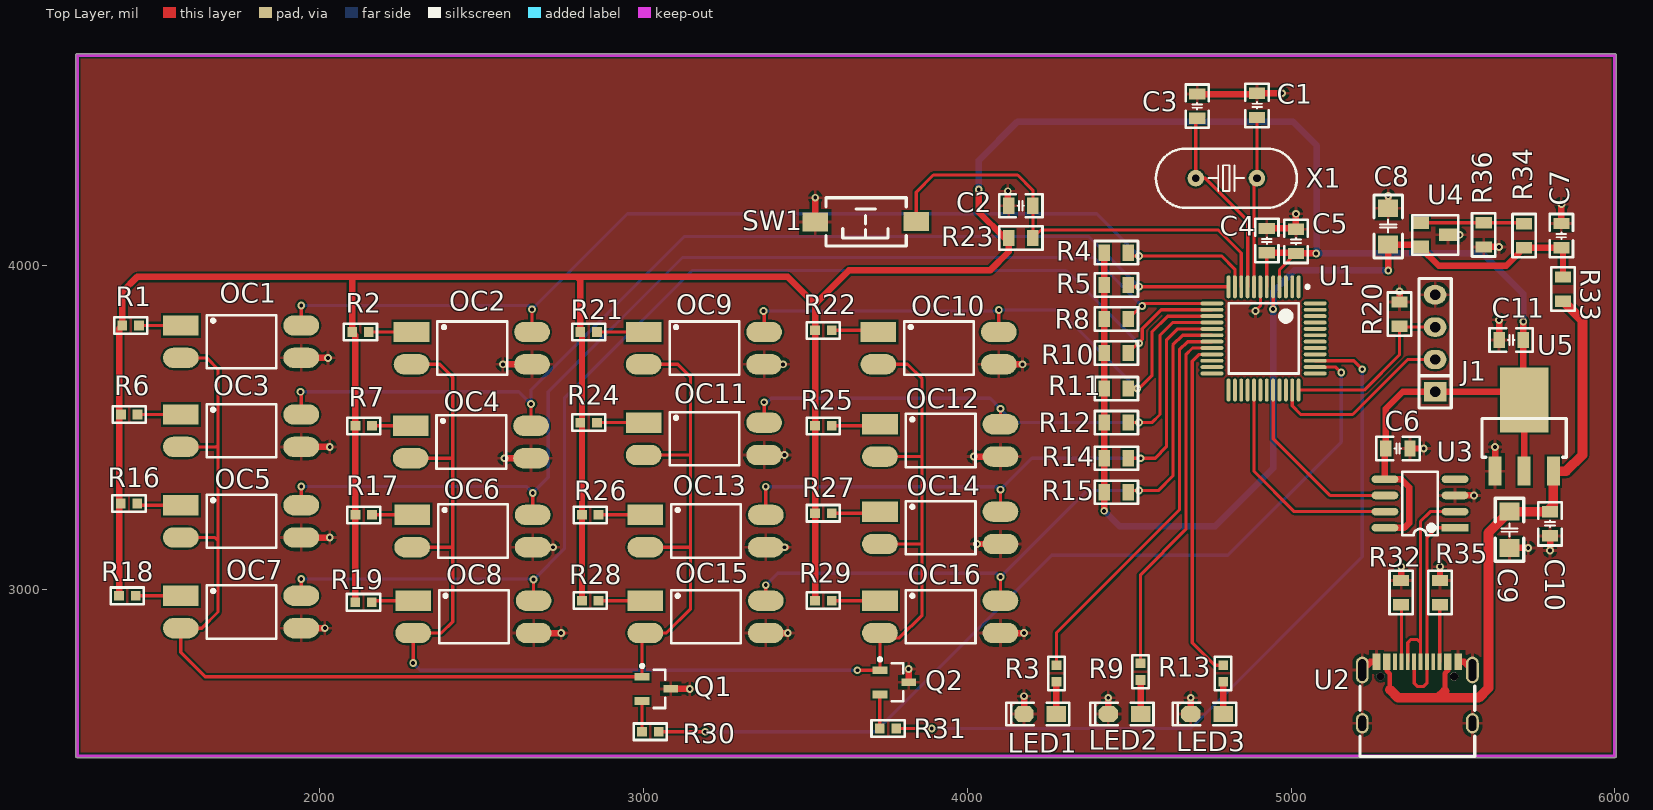
[diagram p0: Top Layer view]
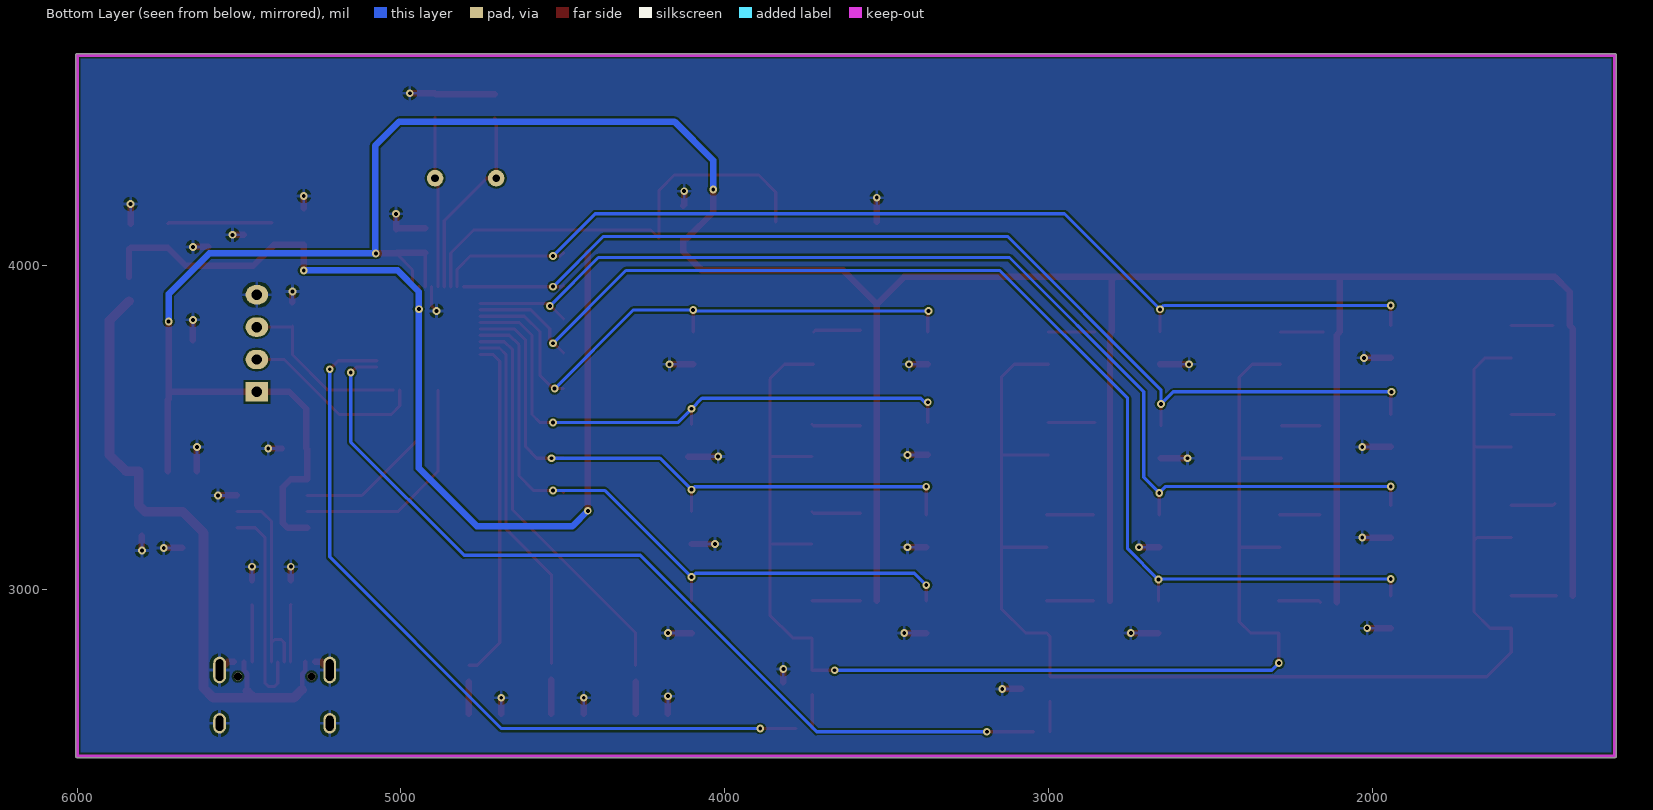
[diagram p1: Bottom Layer view, seen from below]
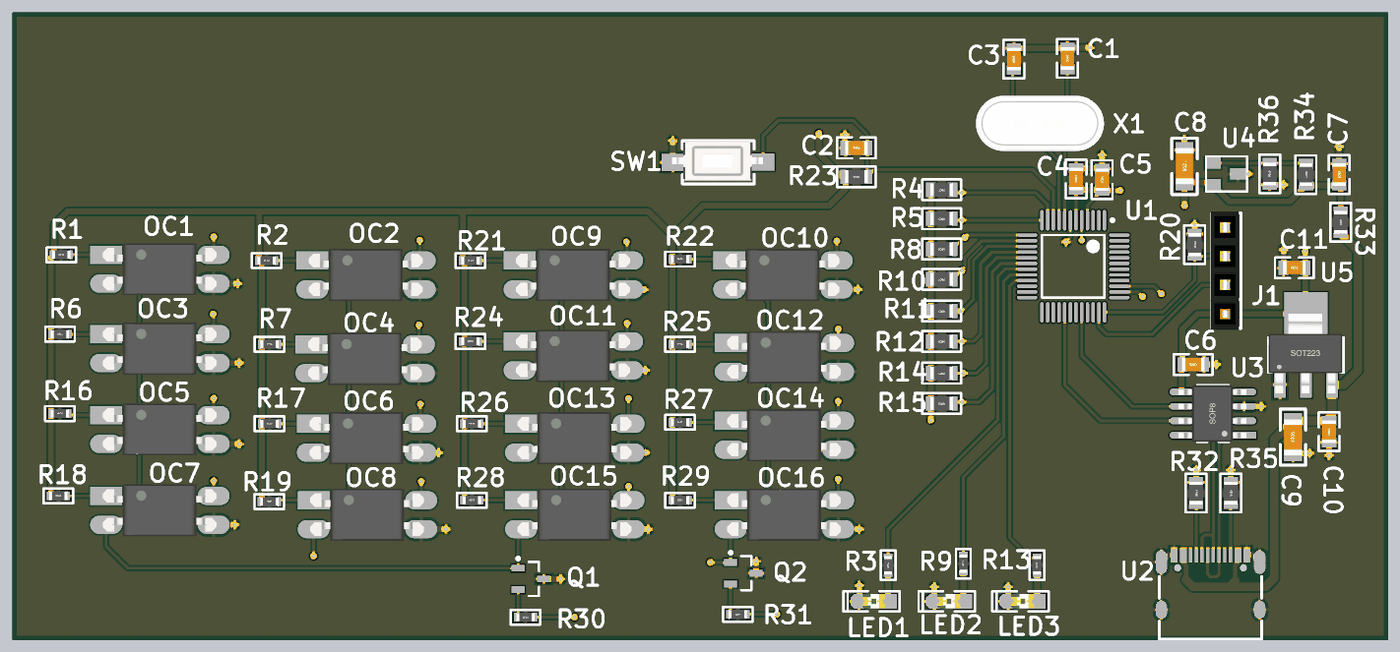
[diagram p2: 3D render of the assembled board from above, using the file's embedded part models]
# Altium PCB MISC82094.PcbDoc
Units mil, origin at the board's own origin, x right, y up, seen from the top; angles counter-clockwise.
Board outline 4760.03 x 2175.03 mil, 2 copper layers (Top Layer, Bottom Layer); 76 components, 52 nets, 259 pads, 75 vias.

## Layer stack, top to bottom (the 12.6 mil dielectric is the usual default, probably not edited)
Top Solder: solder mask 0.4, Solder Resist, Dk 3.5
Top Layer: signal copper 1.4
Dielectric 1: dielectric 12.6, FR-4, Dk 4.8
Bottom Layer: signal copper 1.4
Bottom Solder: solder mask 0.4, Solder Resist, Dk 3.5

## Board outline
1250,2479.99 cw(c1250,2485) 1244.98,2485 1244.98,4650 cw(c1250,4650) 1250,4655.02 6000,4655.02 cw(c6000,4650) 6005.02,4650 6005.02,2485 cw(c6000,2485) 6000,2479.99

## Design rules (kind name [scope] priority, off if disabled: settings)
Clearance [All] p1: gap=6
MinimumSolderMaskSliver [All] p1: minsoldermaskwidth=0
PolygonConnect [All] p1: connectstyle=Relief reliefconductorwidth=10 reliefentries=4 polygonreliefangle="90 Angle" airgapwidth=10
RoutingVias [All] p1: holewidth=28 width=50 viastyle="Through Hole" minholewidth=28 minwidth=50 maxholewidth=28 maxwidth=50
SilkToSilkClearance [All] p1: silktosilkclearance=0
SilkToSolderMaskClearance [IsPad] p1: minsilkscreentomaskgap=0 clearancetoexposedcopper=TRUE
SolderMaskExpansion [All] p1: expansion=4
Width [All] p1: maxlimit=50 minlimit=10 preferedwidth=10
27 further rules are at their usual default settings.

## Components (designator, comment, footprint, x,y, rotation, side; value= is the part's Value field where it differs from the comment)
C1 "22PF" "C 0805_L" 4895,4495 r270 top
C2 "0.1UF" "C 0805_L" 4165,4185 r0 top
C3 "22PF" "C 0805_L" 4710,4492.6 r90 top
C4 "0.1UF" "C 0805_L" 4925,4077.4 r270 top
C5 "0.1UF" "C 0805_L" 5015,4075 r270 top
C6 "0.1UF" "C 0805_L" 5330,3435 r180 top
C7 "0.1UF" "C 0805_L" 5835,4092.6 r270 top
C8 "10UF" "C 1206_L" 5300,4122.09 r270 top
C9 "30UF" "C 1206_L" 5675,3182.91 r90 top
C10 "0.1UF" "C 0805_L" 5800,3202.4 r90 top
C11 "0.1UF" "C 0805_L" 5680,3770 r0 top
J1 "Female HDR1X4" Fe-HDR1X4/2.54-S 5445,3610 r180 top
LED1 "Red" "LED 0805G" 4225,2615 r180 top
LED2 "Red" "LED 0805G" 4485,2615 r180 top
LED3 "Red" "LED 0805G" 4740,2615 r180 top
OC1 "ITR20001" SMD_PC817 1570,3815 r0 top
OC2 "ITR20001" SMD_PC817 2282.88,3795 r0 top
OC3 "ITR20001" SMD_PC817 1570,3540 r0 top
OC4 "ITR20001" SMD_PC817 2280,3505 r0 top
OC5 "ITR20001" SMD_PC817 1570,3260 r0 top
OC6 "ITR20001" SMD_PC817 2285,3230 r0 top
OC7 "ITR20001" SMD_PC817 1570,2980 r0 top
OC8 "ITR20001" SMD_PC817 2287.88,2965 r0 top
OC9 "ITR20001" SMD_PC817 3000,3795 r0 top
OC10 "ITR20001" SMD_PC817 3725,3795 r0 top
OC11 "ITR20001" SMD_PC817 3000,3515 r0 top
OC12 "ITR20001" SMD_PC817 3730,3510 r0 top
OC13 "ITR20001" SMD_PC817 3005,3230 r0 top
OC14 "ITR20001" SMD_PC817 3730,3240 r0 top
OC15 "ITR20001" SMD_PC817 3005,2965 r0 top
OC16 "ITR20001" SMD_PC817 3730,2965 r0 top
Q1 "QNPN" SOT-23B_N 3039.29,2692.4 r0 top
Q2 "QNPN" SOT-23B_N 3774.29,2712.6 r0 top
R1 "330" "R 0603_L" 1415,3815 r0 top
R2 "330" "R 0603_L" 2125,3795 r0 top
R3 "330" "R 0603_L" 4275,2740 r90 top
R4 "10K" "R 0805_L" 4460,4040 r180 top
R5 "10K" "R 0805_L" 4460,3940 r180 top
R6 "330" "R 0603_L" 1410.59,3540 r0 top
R7 "330" "R 0603_L" 2135,3505 r0 top
R8 "10K" "R 0805_L" 4460,3835 r180 top
R9 "330" "R 0603_L" 4535,2745.59 r90 top
R10 "10K" "R 0805_L" 4460,3730 r180 top
R11 "10K" "R 0805_L" 4460,3620 r180 top
R12 "10K" "R 0805_L" 4460,3515 r180 top
R13 "330" "R 0603_L" 4790,2740 r90 top
R14 "10K" "R 0805_L" 4460,3405 r180 top
R15 "10K" "R 0805_L" 4460,3300 r180 top
R16 "330" "R 0603_L" 1410,3265 r0 top
R17 "330" "R 0603_L" 2135,3230 r0 top
R18 "330" "R 0603_L" 1405,2980 r0 top
R19 "330" "R 0603_L" 2134.41,2960 r0 top
R20 "10K" "R 0805_L" 5335,3850 r270 top
R21 "330" "R 0603_L" 2830,3795 r0 top
R22 "330" "R 0603_L" 3555,3800 r0 top
R23 "10K" "R 0805_L" 4165,4085 r180 top
R24 "330" "R 0603_L" 2830,3515 r0 top
R25 "330" "R 0603_L" 3555,3505 r0 top
R26 "330" "R 0603_L" 2835,3230 r0 top
R27 "330" "R 0603_L" 3555,3235 r0 top
R28 "330" "R 0603_L" 2835,2965 r0 top
R29 "330" "R 0603_L" 3555,2965 r0 top
R30 "330" "R 0603_L" 3020.59,2560 r180 top
R31 "330" "R 0603_L" 3755,2570 r180 top
R32 "5.1K" "R 0805_L" 5340,2990 r270 top
R33 "330" "R 0805_L" 5840,3927.6 r270 top
R34 "3.3K" "R 0805_L" 5720,4092.4 r270 top
R35 "5.1K" "R 0805_L" 5460,2990 r270 top
R36 "10K" "R 0805_L" 5595,4095 r90 top
SW1 "3x6x5" "TSW SMD-3*6*2.5" 3685,4135 r180 top
U1 "STM32G030C8T6" LQFP48_N 4915,3775 r270 top
U2 "HC-TYPE-C-16P-01A COPY" USB-C-SMD_HC-TYPE-C-16P-01A 5390,2640 r0 top
U3 "CH340N" SOP8 5506.54,3190 r180 top
U4 "TL431DBZ" SOT-23 5445.63,4095 r270 top
U5 "AMS1117" SOT223 5720,3365 r0 top
X1 "12MHz" "OSC HC-49S" 4800,4270 r0 top

## Footprints (in the part's own frame and the unit in brackets; to place one, negate y for a bottom-side part, rotate by r counter-clockwise, add the part's x,y. Pads: shape width x height; smd on the part's side, far side on the other; paste and mask are expansions set on the pad)
"C 0805_L" [mil] "无极性贴片电容"
  rect 35x50 smd: 1(-37.4,0) 2(37.4,0)
  silkscreen extent -67,-36 67,36, body extent -39,-24 39,24, height 20
"C 1206_L" [mil] "无极性贴片电容"
  rect 55x62 smd: 1(-55.12,0) 2(57.09,0)
  silkscreen extent -96,-44 98,44, body extent -63,-32 63,32, height 48
Fe-HDR1X4/2.54-S [mil]
  rect 70x60 hole 32: 1(0,0)
  oval 70x60 hole 32: 2(0,-100) 3(0,-200) 4(0,-300)
  silkscreen extent -50,-350 50,50, body extent -44,-355 54,55, height 335
"LED 0805G" [mil] "绿色0805LED"
  rect 60x50 smd: 1(-50,0)
  oct 60x50 smd: 2(50,0)
  silkscreen extent -90,-35 105,35, body extent -39,-25 39,25, height 32
LQFP48_N [mm] "Thin QFP, 48-Leads, Body 7x7mm, Pitch 0.5mm, IPC Medium Density"
  oval 1.8x0.3 smd: 1(-4.05,2.75) 2(-4.05,2.25) 3(-4.05,1.75) 4(-4.05,1.25) 5(-4.05,0.75) 6(-4.05,0.25) 7(-4.05,-0.25) 8(-4.05,-0.75) 9(-4.05,-1.25) 10(-4.05,-1.75) 11(-4.05,-2.25) 12(-4.05,-2.75) 25(4.05,-2.75) 26(4.05,-2.25) 27(4.05,-1.75) 28(4.05,-1.25) 29(4.05,-0.75) 30(4.05,-0.25) 31(4.05,0.25) 32(4.05,0.75) 33(4.05,1.25) 34(4.05,1.75) 35(4.05,2.25) 36(4.05,2.75)
  oval 0.3x1.8 smd: 13(-2.75,-4.05) 14(-2.25,-4.05) 15(-1.75,-4.05) 16(-1.25,-4.05) 17(-0.75,-4.05) 18(-0.25,-4.05) 19(0.25,-4.05) 20(0.75,-4.05) 21(1.25,-4.05) 22(1.75,-4.05) 23(2.25,-4.05) 24(2.75,-4.05) 37(2.75,4.05) 38(2.25,4.05) 39(1.75,4.05) 40(1.25,4.05) 41(0.75,4.05) 42(0.25,4.05) 43(-0.25,4.05) 44(-0.75,4.05) 45(-1.25,4.05) 46(-1.75,4.05) 47(-2.25,4.05) 48(-2.75,4.05)
  silkscreen extent -4.17,-2.75 2.75,3.58, body extent -3.5,-3.5 3.5,3.5, height 1.6
"OSC HC-49S" [mm]
  round 1.3 hole 0.6: 1(-2.4,0) 2(2.4,0)
  silkscreen extent -5.52,-2.32 5.52,2.33, body extent -5.52,-2.32 5.53,2.33, height 4.13
"R 0603_L" [mil] "1/10W贴片电阻"
  rect 30x30 smd: 1(-25.59,0) 2(25.59,0)
  silkscreen extent -51,-26 51,26, body extent -31,-16 32,16, height 16
"R 0805_L" [mil] "1/8W贴片电阻"
  rect 35x50 smd: 1(-37.4,0) 2(37.4,0)
  silkscreen extent -67,-36 67,36, body extent -39,-25 39,25, height 20
SMD_PC817 [mm]
  rect 2.8x1.6 smd mask+0: 1(0,0)
  oval 2.8x1.6 smd mask+0: 2(0,-2.54) 3(9.452,-2.54) 4(9.452,0)
  silkscreen extent 2.03,-3.36 7.49,0.82, body extent -0.3,-3.56 9.7,1.02, height 3.85
SOP8 [mm]
  rect 2.1x0.6 smd: 1(0,0)
  oval 2.1x0.6 smd: 2(0,-1.27) 3(0,-2.54) 4(0,-3.81) 5(5.5,-3.81) 6(5.5,-2.54) 7(5.5,-1.27) 8(5.5,0)
  silkscreen extent 1.35,-4.41 4.15,0.6, body extent -0.21,-4.4 5.8,0.6, height 1.9
SOT223 [mil]
  rect 40x90 smd: 1(-90,0) 2(0,0) 3(90,0)
  rect 150x200 smd: 2(0,220)
  silkscreen extent -130,43 130,163, body extent -130,-30 126,246, height 65
SOT-23 [mm]
  rect 1x1.4 smd paste+0 mask+0.051: 1(-0.95,-1.2) 2(0.95,-1.2) 3(0,1)
  silkscreen extent -1.55,-1.8 1.55,1.8
SOT-23B_N [mm] "SOT23, 3-Leads, Body 2.9x1.3mm, Pitch 0.95mm, Lead Span 2.4mm, IPC Medium Density"
  rect 1.15x0.6 smd: 1(-1.125,0.95) 2(-1.125,-0.95) 3(1.125,0)
  silkscreen extent -1.25,-1.5 0.7,1.92, body extent -0.7,-1.5 0.7,1.5, height 1.14
"TSW SMD-3*6*2.5" [mm] "3*6*2.5mm"
  rect 2x1.5 smd: 1(-3.996,-0.02) 2(3.937,0)
  silkscreen extent -3.21,-1.9 3.09,1.9, body extent -4,-1.88 4,1.62, height 2.59
USB-C-SMD_HC-TYPE-C-16P-01A [mm]
  oval 1x2.1 hole 0.6 slot 1.7 at 90 deg paste+0 mask+0.05: 1(-4.32,2.809) 2(4.32,2.809)
  oval 1x1.6 hole 0.6 slot 1.2 at 90 deg paste+0 mask+0.05: 3(4.32,-1.372) 4(-4.32,-1.372)
  rect 0.6x1.3 smd paste-100 mask+0.05: A1B12(-3.2,3.448) A4B9(-2.4,3.448) B1A12(3.2,3.448) B4A9(2.4,3.448)
  rect 0.3x1.3 smd paste-100 mask+0.05: A5(-1.25,3.448) A6(-0.25,3.448) A7(0.25,3.448) A8(1.25,3.448) B5(1.75,3.448) B6(0.75,3.448) B7(-0.75,3.448) B8(-1.75,3.448)
  round 0.65 hole 0.65 unplated paste+0: ""(-2.89,2.308) ""(2.89,2.308)
  silkscreen extent -4.5,-3.97 4.5,1.55

## Part data
C1 C2 C3 C4 C5 C6 C7 C8 C9 C10 C11: library part C, "SMD capacitor"
LED1 LED2 LED3: library part LED-SMD, "SMD LED"
OC1 OC2 OC3 OC4 OC5 OC6 OC7 OC8 OC9 OC10 OC11 OC12 OC13 OC14 OC15 OC16: library part PC817, "Linear optocoupler"
Q1 Q2: "NPN Bipolar Transistor"
R1 R2 R3 R4 R5 R6 R7 R8 R9 R10 R11 R12 R13 R14 R15 R16 R17 R18 R19 R20 R21 R22 R23 R24 R25 R26 R27 R28 R29 R30 R31 R32 R33 R34 R35 R36: library part R, "SMD resistor"
SW1: library part "TSW 3x6", "3x6 tact switch"
U5: "Three-terminal voltage regulator"
X1: library part XTAL-2P, "2-pin passive crystal oscillator"

## Via types
v1: diameter 24, hole 12, Top Layer to Bottom Layer, 75 vias

## Nets (pads, with @x,y where several pads share a name; then routed paths per layer and width w, separated by ;. In a path a pad name is that pad's centre, name@x,y a point inside that pad or via, vN(x,y) a via of type N, cw(c..) or ccw(c..) an arc to the next point about the centre after c; other vN are vias at no path point)
ADC_IN0: OC1.4 OC2.4 R4.1 U1.11 | length 3305.5
  Top Layer w10: OC1.4 v1(1942.12,3877.12) ; OC2.4 v1(2655,3865) ; R4.1 4507.41,4030 v1(4530,4030) 4785,4030 4826.42,3988.58 U1.11
  Bottom Layer w10: v1(1942.12,3877.12) 2642.88,3877.12 v1(2655,3865) 2950,4160 4400,4160 v1(4530,4030)
ADC_IN1: OC3.4 OC4.4 R5.1 U1.12 | length 3357.4
  Top Layer w10: OC3.4 v1@1942.12,3607.88 ; OC4.4 v1(2652.12,3572.12) ; R5.1 4502.96,3934.45 U1.12
  Bottom Layer w10: v1(1940,3610) 2614.24,3610 v1(2652.12,3572.12) 2652.12,3617.12 3125,4090 4375,4090 v1(4530,3935)
ADC_IN2: OC5.4 OC6.4 R8.1 U1.13 | length 3528.2
  Top Layer w10: OC5.4 v1(1942.12,3317.88) ; OC6.4 v1(2657.12,3297.88) ; R8.1 4545.67,3883.27 U1.13
  Bottom Layer w10: v1(1942.12,3317.88) 2637.12,3317.88 v1(2657.12,3297.88) 2705,3345.76 2705,3610 3120,4025 4390,4025 v1(4540,3875)
ADC_IN3: OC7.4 OC8.4 R10.1 U1.14 | length 3799.5
  Top Layer w10: OC7.4 v1(1942.12,3032.12) ; OC8.4 v1(2660,3030) ; R10.1 4540,3772.6 4540,3805 4598.58,3863.58 U1.14
  Bottom Layer w10: v1(1942.12,3032.12) 2657.88,3032.12 v1(2660,3030) 2755,3125 2755,3590 3150,3985 4305,3985 v1(4530,3760)
ADC_IN4: OC9.4 OC10.4 R11.1 U1.15 | length 1817.5
  Top Layer w10: OC9.4 v1@3372.12,3857.88 ; OC10.4 v1(4097.12,3862.88) ; R11.1 4530,3620 4570,3660 4570,3795 4618.9,3843.9 U1.15
  Bottom Layer w10: v1(3370,3860) 4094.24,3860 v1(4097.12,3862.88) 4282.12,3862.88 v1(4525,3620)
ADC_IN5: OC11.4 OC12.4 R12.1 U1.16 | length 1834.5
  Top Layer w10: OC11.4 v1(3372.12,3577.88) ; OC12.4 v1(4102.12,3557.88) ; R12.1 4570,3515 4595,3540.01 4595,3785 4634.21,3824.21 U1.16
  Bottom Layer w10: v1(3372.12,3577.88) 3382.12,3577.88 3394.24,3590 4070,3590 v1(4102.12,3557.88) 4145,3515 v1(4530,3515)
ADC_IN6: OC13.4 OC14.4 R14.1 U1.17 | length 1973.9
  Top Layer w10: OC13.4 v1(3377.12,3317.12) ; OC14.4 v1(4102.12,3307.88) ; R14.1 4580,3405 4615,3440 4615,3770 4649.53,3804.53 U1.17
  Bottom Layer w10: v1(3377.12,3317.12) 4092.88,3317.12 v1(4102.12,3307.88) 4199.24,3405 v1(4535,3405)
ADC_IN7: OC15.4 OC16.4 R15.1 U1.18 | length 2100.9
  Top Layer w10: OC15.4 v1(3377.12,3012.88) ; OC16.4 v1(4102.12,3037.88) ; R15.1 4502.4,3305 v1(4530,3305) 4590,3305 4635,3350 4635,3755 4664.84,3784.84 U1.18
  Bottom Layer w10: v1(3377.12,3012.88) 3414.24,3050 4090,3050 v1(4102.12,3037.88) 4369.24,3305 v1(4530,3305)
BANK0: R30.1 U1.38 | length 2781.9
  Top Layer w10: R30.1 v1(3190,2560) ; U1.38 5138.58,3686.42 v1(5155,3670)
  Bottom Layer w10: v1(3190,2560) 3715,2560 4260,3105 4805,3105 5155,3455 v1(5155,3670)
BANK1: R31.1 U1.39 | length 2395.3
  Top Layer w10: R31.1 v1(3890,2570) ; U1.39 5193.9,3706.1 v1(5220,3680)
  Bottom Layer w10: v1(3890,2570) 4690,2570 5220,3100 v1(5220,3680)
GND: C1.1 C2.1 C3.2 C4.1 C5.1 C6.1 C7.1 C8.1 C9.1 C10.1 C11.1 J1.4 LED1.2 LED2.2 LED3.2 OC1.3 OC2.3 OC3.3 OC4.3 OC5.3 OC6.3 OC7.3 OC8.3 OC9.3 OC10.3 OC11.3 OC12.3 OC13.3 OC14.3 OC15.3 OC16.3 Q1.3 Q2.3 R20.1 R32.1 R35.1 R36.1 SW1.2 U1.7 U2.1 U2.2 U2.3 U2.4 U2.A1B12 U2.B1A12 U3.3 U4.3 U5.1 | length 2825.1
  Top Layer w10: v1(4890,3860) 4905.16,3875.16 U1.7
  Top Layer w20: OC7.3 v1(2015,2880) ; OC5.3 v1(2030,3160) ; OC3.3 v1(2030,3440) ; OC1.3 v1(2025,3715) ; v1(2565,3695) OC2.3 ; v1(2570,3405) OC4.3 ; OC6.3 v1(2720,3130) ; OC8.3 v1@2750,2865 ; Q1.3 v1(3142.4,2692.4) ; OC11.3 v1(3435,3415) ; OC9.3 v1(3430,3695) ; OC15.3 v1(3445,2865) ; OC13.3 v1@3440,3130 ; SW1.2 v1(3530,4210) ; Q2.3 v1(3818.58,2753.58) ; v1(4020,3410) OC12.3@4112.12,3410 ; v1(4030,3140) OC14.3 ; OC10.3 v1(4170,3695) ; OC16.3 v1(4175,2865) ; v1(4125,4230) 4125,4187.59 C2.1 ; LED1.2 v1(4175,2670) ; LED2.2 v1(4435,2665) ; LED3.2 v1(4690,2665) ; C3.2 4892.59,4530 C1.1 v1(4972.4,4532.4) ; C4.1 5012.6,4114.8 C5.1 v1(5015,4160) ; U2.1 5245.1,2775.76 U2.A1B12 ; C8.1 v1(5300,4215) ; R20.1 v1(5335,3920) ; R32.1 v1(5340,3070) ; C6.1 v1(5410,3435) ; R35.1 v1(5460,3070) ; U4.3 v1(5520,4095) ; U3.3 v1(5565,3290) ; U2.B1A12 5534.89,2775.76 U2.2 ; R36.1 v1(5642.6,4057.6) ; U5.1 v1(5630,3440) ; C11.1 v1(5642.6,3832.4) ; C9.1 v1(5732.8,3127.8) ; v1(5800,3120) C10.1 ; C7.1 v1(5835,4190)
  other v1: 2745,2865 3435,3130
NetC1_2: C1.2 U1.8 X1.2 | length 527.1
  Top Layer w10: U1.8 4885.47,4260.98 X1.2 4894.49,4457.09 C1.2
NetC2_2: C2.2 R23.1 SW1.1 U1.10 | length 1428.6
  Top Layer w10: SW1.1 3842.31,4227.31 3895,4280 4155,4280 4202.4,4232.6 R23.1 4227.4,4110 4775,4110 4846.1,4038.9 U1.10
NetC3_1: C3.1 U1.9 X1.1 | length 606.3
  Top Layer w10: C3.1 4705.51,4450.71 X1.1 4735,4270 4865.79,4139.21 U1.9
NetLED1_1: LED1.1 R3.1 | length 99.4
  Top Layer w20: LED1.1 R3.1
NetLED2_1: LED2.1 R9.1 | length 105
  Top Layer w20: LED2.1 R9.1
NetLED3_1: LED3.1 R13.1 | length 99.4
  Top Layer w20: LED3.1 R13.1
NetOC1_1: OC1.1 R1.2 | length 129.4
  Top Layer w10: R1.2 OC1.1
NetOC1_2: OC1.2 OC3.2 OC5.2 OC7.2 OC9.2 OC11.2 OC13.2 OC15.2 Q1.1 | length 4256.6
  Top Layer w10: OC5.2 1675,3160 1685,3150 ; OC3.2 1680,3440 1685,3445 ; OC1.2 1650,3715 1685,3680 1685,3445 ; OC11.2 3145,3415 ; OC9.2 3105,3695 3145,3655 3145,3415 ; OC13.2 3140,3130 3145,3135 ; 1685,3150 1685,3445 ; 1685,3150 1685,2930 1635,2880 OC7.2 1570,2805 1645.2,2729.8 Q1.1 2995,2855 OC15.2 3070,2865 3145,2940 3145,3135 ; 3145,3135 3145,3415
NetOC2_1: OC2.1 R2.2 | length 132.3
  Top Layer w10: R2.2 OC2.1
NetOC2_2: OC2.2 OC4.2 OC6.2 OC8.2 OC10.2 OC12.2 OC14.2 OC16.2 Q2.1 | length 4241.2
  Top Layer w10: OC4.2 2405,3405 2410,3410 ; OC2.2 2370,3695 2410,3655 2410,3410 ; OC6.2 2410,3130 ; v1(2287.88,2772.12) OC8.2 2375,2865 2410,2900 2410,3130 ; v1(3660,2750) Q2.1 3730,2850 3790,2850 3860,2920 3860,3140 ; OC10.2 3815,3695 3860,3650 3860,3415 ; OC14.2 3860,3140 ; OC12.2 3855,3410 3860,3415 ; 2410,3130 2410,3410 ; 3860,3140 3860,3415
  Bottom Layer w10: v1(2287.88,2772.12) 2310,2750 v1(3660,2750)
NetOC3_1: OC3.1 R6.2 | length 133.8
  Top Layer w10: R6.2 OC3.1
NetOC4_1: OC4.1 R7.2 | length 119.4
  Top Layer w10: R7.2 OC4.1
NetOC5_1: OC5.1 R16.2 | length 136.5
  Top Layer w10: R16.2 1440.58,3260 OC5.1
NetOC6_1: OC6.1 R17.2 | length 124.4
  Top Layer w10: R17.2 OC6.1
NetOC7_1: OC7.1 R18.2 | length 139.4
  Top Layer w10: R18.2 OC7.1
NetOC8_1: OC8.1 R19.2 | length 130
  Top Layer w10: R19.2 2165,2965 OC8.1
NetOC9_1: OC9.1 R21.2 | length 144.4
  Top Layer w10: R21.2 OC9.1
NetOC10_1: OC10.1 R22.2 | length 146.5
  Top Layer w10: R22.2 3720,3800 OC10.1
NetOC11_1: OC11.1 R24.2 | length 144.4
  Top Layer w10: R24.2 OC11.1
NetOC12_1: OC12.1 R25.2 | length 151.5
  Top Layer w10: R25.2 3725,3505 OC12.1
NetOC13_1: OC13.1 R26.2 | length 144.4
  Top Layer w10: R26.2 OC13.1
NetOC14_1: OC14.1 R27.2 | length 151.5
  Top Layer w10: R27.2 3725,3235 OC14.1
NetOC15_1: OC15.1 R28.2 | length 144.4
  Top Layer w10: R28.2 OC15.1
NetOC16_1: OC16.1 R29.2 | length 149.4
  Top Layer w10: R29.2 OC16.1
NetQ1_2: Q1.2 R30.2 | length 95
  Top Layer w10: R30.2 Q1.2
NetQ2_2: Q2.2 R31.2 | length 105.4
  Top Layer w10: R31.2 3729.41,2674.61 Q2.2
NetR3_2: R3.2 U1.19 | length 1242.8
  Top Layer w10: R3.2 4275,2865 4655,3245 4655,3740 4680.16,3765.16 U1.19
NetR9_2: R9.2 U1.20 | length 1100.8
  Top Layer w10: R9.2 4535,3045 4675,3185 4675,3725 4695.47,3745.47 U1.20
NetR13_2: R13.2 U1.21 | length 1062.9
  Top Layer w10: U1.21 4715.79,3725.79 4695,3705 4695,2835 4764.41,2765.59 R13.2
NetR32_2: R32.2 U2.A5 | length 177.2
  Top Layer w10: R32.2 5340.79,2951.81 U2.A5
NetR34_1: R34.1 R36.2 U4.1 | length 322.7
  Top Layer w10: U4.1 R36.2 5717.4,4132.4 R34.1
NetR35_2: R35.2 U2.B5 | length 177.3
  Top Layer w10: U2.B5 5458.9,2951.5 R35.2
NetU2_A6: U2.A6 U2.B6 U3.1 | length 662.9
  Top Layer w10: U2.A6 5380.16,2709.84 5390,2700 5410,2700 5419.53,2709.53 U2.B6 5419.53,3159.53 5450,3190 U3.1
NetU2_A7: U2.A7 U2.B7 U3.2 | length 660.4
  Top Layer w10: U2.B7 5360.47,2835.47 5370,2845 5390,2845 5399.84,2835.16 ; U2.A7 5399.84,2835.16 ; U3.2 5430,3240 5399.84,3209.84 5399.84,2835.16
SWCLK: J1.3 R20.2 U1.36 | length 555.7
  Top Layer w10: U1.36 5225.55,3615.55 5335,3725 R20.2 5337.6,3810 J1.3
SWDIO: J1.2 U1.35 | length 571.9
  Top Layer w10: U1.35 5003.58,3566.42 5030,3540 5190,3540 5360,3710 J1.2
UART_RX: U1.32 U3.6 | length 568.2
  Top Layer w10: U1.32 4944.53,3465.47 5120,3290 U3.6
UART_TX: U1.29 U3.7 | length 707.1
  Top Layer w10: U1.29 4885.47,3364.53 5010,3240 U3.7
VBUS: C9.2 C10.2 R33.2 U2.A4B9 U2.B4A9 U5.3 | length 1971.4
  Top Layer w15: U2.A4B9 5295.51,2748.78 5305,2739.29 5305,2690 ; 5475,2685 5475,2740 5484.49,2749.49 U2.B4A9
  Top Layer w30: 5305,2690 5330,2665 5455,2665 ; 5475,2685 5455,2665 ; R33.2 5900,3830.2 5900,3415 5850,3365 U5.3 5810,3260 5790,3240 C9.2 5610,3175 5610,2695 5580,2665 5455,2665
VCC: C4.2 C5.2 C6.2 C11.2 J1.1 R1.1 R2.1 R6.1 R7.1 R16.1 R17.1 R18.1 R19.1 R21.1 R22.1 R23.2 R24.1 R25.1 R26.1 R27.1 R28.1 R29.1 U1.4 U1.6 U3.5 U3.8 U5.2 | length 11088
  Top Layer w10: U1.6 4924.84,4039.84 C4.2 ; U1.4 4964.21,3986.82 C5.2
  Top Layer w20: R18.1 1379.41,3805 R1.1 1389.41,3919.41 1435,3965 2095,3965 ; R19.1 2108.82,3785.58 R2.1 2099.41,3960.59 2095,3965 ; R28.1 R26.1 2809.41,3790 R21.1 2804.41,3955.59 2795,3965 ; R29.1 R27.1 R25.1 R22.1 3529.41,3880.59 ; v1(4035,4235) 4035,4165 4115,4085 R23.2 4127.6,4042.6 4070,3985 3633.81,3985 3529.41,3880.59 ; C4.2 5012.6,4040 C5.2 v1(5077.4,4037.6) ; U3.8 5350.3,3190 5365,3204.7 5365,3315 5340,3340 U3.5 5290,3432.4 C6.2 5292.6,3557.6 5345,3610 J1.1 U5.2@5717.4,3610 ; v1(5717.4,3827.4) C11.2 U5.2@5717.4,3610 ; U5.2@5720,3365 5720,3585 5717.4,3587.6 U5.2@5717.4,3610 ; 2095,3965 2795,3965 ; 2795,3965 3445,3965 3529.41,3880.59
  Bottom Layer w20: v1(4035,4235) 4035,4325 4155,4445 5005,4445 5080,4370 5080,4040.2 v1(5077.4,4037.6) 5592.4,4037.6 5717.4,3912.6 v1(5717.4,3827.4)
VREF: C7.2 C8.2 R4.2 R5.2 R8.2 R10.2 R11.2 R12.2 R14.2 R15.2 R33.1 R34.2 U1.5 U4.2 | length 3167.1
  Top Layer w10: v1(4944.53,3865.47) U1.5
  Top Layer w20: v1(4422.6,3242.4) R15.2 R14.2 R12.2 R11.2 R10.2 R8.2 R5.2 R4.2 ; v1(5300,3985) C8.2 5390.99,4065 U4.2 5455.99,4000 5665,4000 R34.2 5834.8,4055 C7.2 5840,4050.2 R33.1
  Bottom Layer w20: v1(4422.6,3242.4) 4470,3195 4765,3195 4944.53,3374.53 v1(4944.53,3865.47) 4944.53,3919.53 5010,3985 v1(5300,3985)
pads on no net: U1.1 U1.2 U1.3 U1.22 U1.23 U1.24 U1.25 U1.26 U1.27 U1.28 U1.30 U1.31 U1.33 U1.34 U1.37 U1.40 U1.41 U1.42 U1.43 U1.44 U1.45 U1.46 U1.47 U1.48 U2. U2.A8 U2.B8 U3.4

## Polygon pours and split planes (outlines as drawn)
GND on Top Layer "D" (solid, remove dead copper, pour order 0): 985,4790 990,4795 6135,4795 6135,2310 6200,2245 6090,2355 1030,2355
GND on Bottom Layer "D" (solid, remove dead copper, pour order 2): 750,4820 6190,4820 6320,4690 6115,4485 6115,2650 6115,2165 6100,2150 5955,2295 920,2295

## Keep-outs
Keep-Out Layer:
  lines w10: 5555,2485 6000,2485 6000,2505 ; 5565,2485 1250,2485 1250,4650 6000,4650 6000,2495